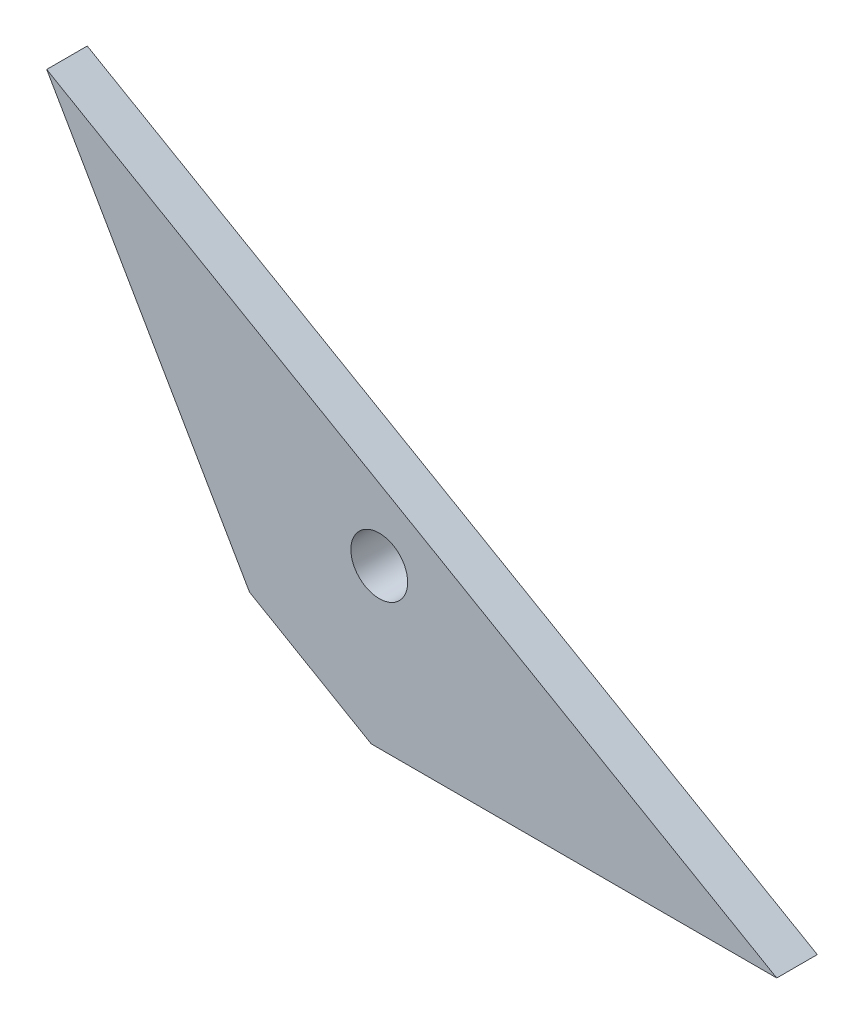
SolidWorks part; units mm, degrees
material "Q235B"
ref_plane "Front Plane" through (0, 0, 0) normal (0, 0, 1) x (1, 0, 0)
ref_plane "Top Plane" through (0, 0, 0) normal (0, 1, 0) x (1, 0, 0)
ref_plane "Right Plane" through (0, 0, 0) normal (1, 0, 0) x (0, 0, -1)
sketch "Sketch1" plane through (0, 0, 0) normal (0, 0, 1) x (1, 0, 0)
  line L0 (-80, 104) -> (-30, 17.3975)
  line L1 (0, 0) -> (100, 0)
  line L3 (100, 0) -> (-80, 104)
  line L5 (-30, 17.3975) -> (0, 0)
  circle A0 centre (2, 39) radius 7
  dimension "D5" = 14
  dimension "D1" = 100
  dimension "D2" = 180
  dimension "D3" = 120
  dimension "D4" = 104
  dimension "D6" = 98
  dimension "D7" = 39
extrude "Boss-Extrude1" add sketch "Sketch1" along normal blind 10
